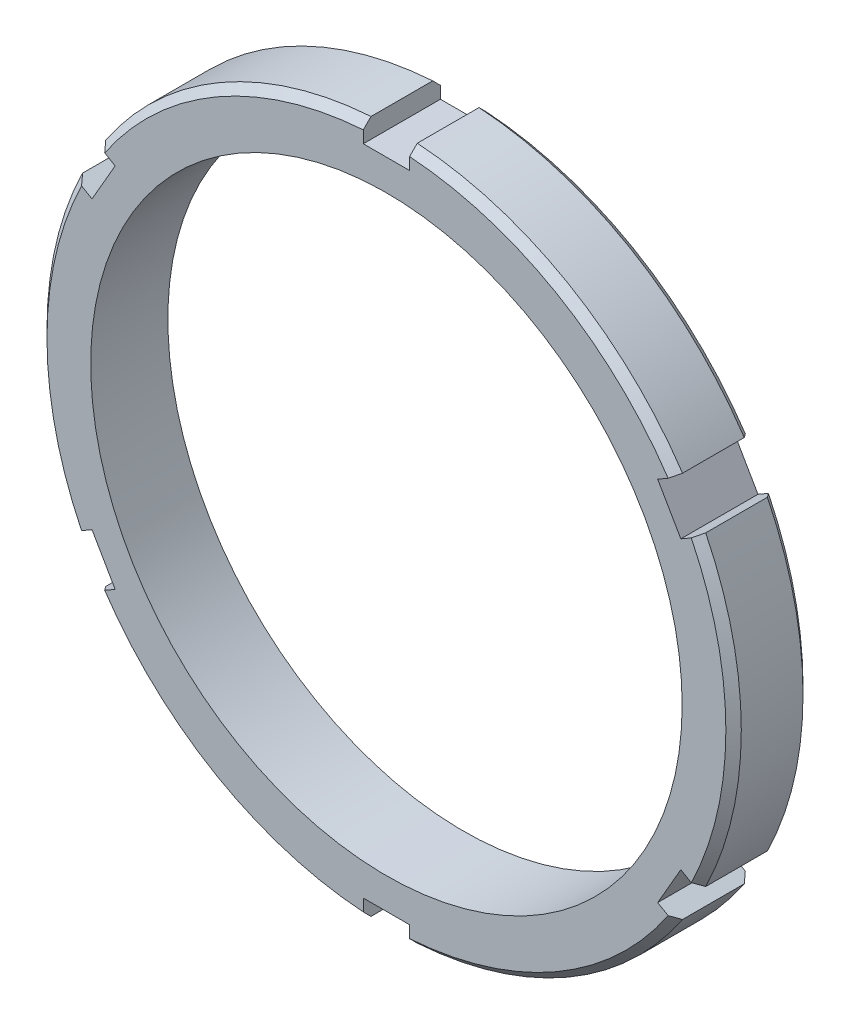
from build123d import *

# Parameters (mm, degrees)
SKETCH1_W          = 30
SKETCH1_H          = 20
CHAMFER1_SIZE      = 3
SKETCH2_W          = 18
SKETCH2_H          = 16
CUT_EXTRUDE1_DEPTH = 38
CIRPATTERN1_COUNT  = 6


with BuildPart() as part:
    # Sketch1 → Revolve1 (revolve)
    with BuildSketch(Plane(origin=(0, 0, 0), x_dir=(0, 0, -1), z_dir=(1, 0, 0)), mode=Mode.PRIVATE) as revolve1_sk:
        with Locations((15, 125)):
            Rectangle(SKETCH1_W, SKETCH1_H)
    revolve(revolve1_sk.sketch.rotate(Axis((0, 0, 0), (0, 0, -1)), 90), axis=Axis((0, 0, 0), (0, 0, -1)))

    # Chamfer1
    chamfer1_edges = [part.edges().sort_by_distance(p)[0] for p in [
        (-135, 0, -30),
        (-135, 0, 0),
    ]]
    chamfer(chamfer1_edges, length=CHAMFER1_SIZE)

    # Sketch2 → Cut-Extrude1 (cut)
    with BuildSketch(Plane.XY):
        with Locations((0, 135)):
            Rectangle(SKETCH2_W, SKETCH2_H)
    cut_extrude1 = extrude(amount=-CUT_EXTRUDE1_DEPTH, mode=Mode.SUBTRACT)

    # CirPattern1: Cut-Extrude1 ×6 about axis
    cirpattern1_axis = Axis((0, 0, 0), (0, 0, 1))
    for i in range(1, CIRPATTERN1_COUNT):
        add(cut_extrude1.rotate(cirpattern1_axis, i * 360 / CIRPATTERN1_COUNT), mode=Mode.SUBTRACT)


solid = part.part
